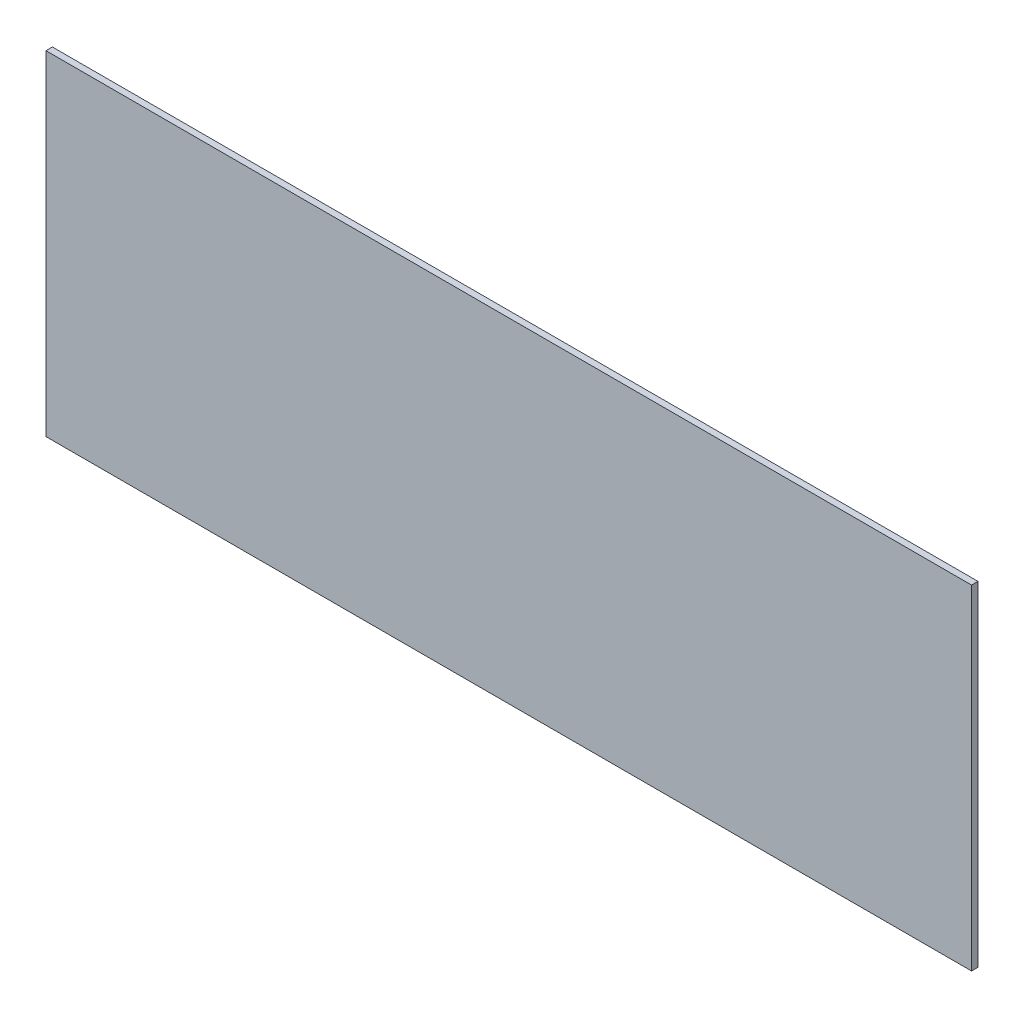
from build123d import *

# Parameters (mm, degrees)
SKETCH_1_W      = 720
SKETCH_1_H      = 260
EXTRUDE_1_DEPTH = 5


with BuildPart() as part:
    # 草图1 → 凸台-拉伸1 (new body)
    with BuildSketch(Plane.XY):
        Rectangle(SKETCH_1_W, SKETCH_1_H)
    extrude(amount=EXTRUDE_1_DEPTH)


solid = part.part
